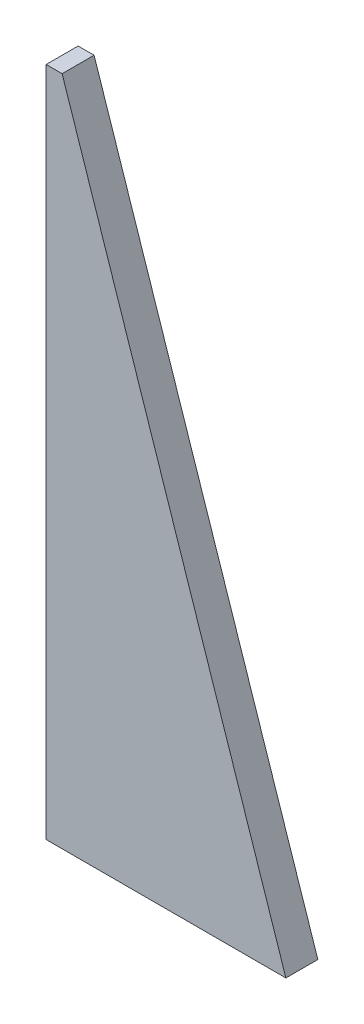
from build123d import *

# Parameters (mm, degrees)
BOSS_EXTRUDE1_DEPTH = 20


with BuildPart() as part:
    # Sketch1 → Boss-Extrude1 (new body)
    with BuildSketch(Plane.XY):
        Polygon((0, 0), (150, 0), (10, 420), (0, 420), align=None)
    extrude(amount=BOSS_EXTRUDE1_DEPTH)


solid = part.part
